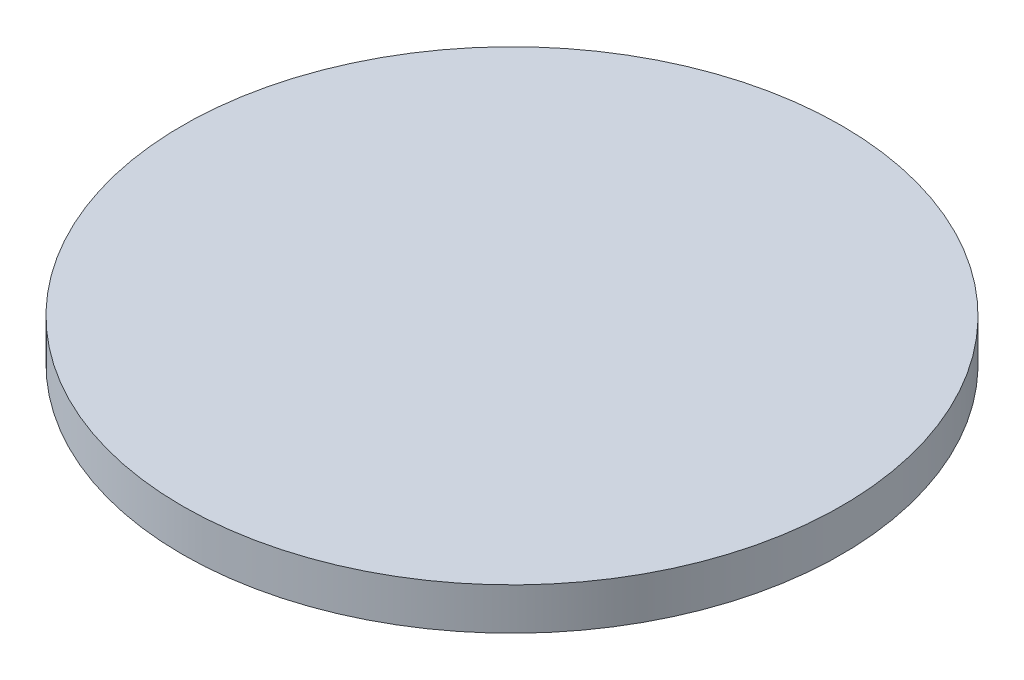
SolidWorks part; units mm, degrees
material "1023 碳钢板 (SS)"
ref_plane "Front Plane" through (0, 0, 0) normal (0, 0, 1) x (1, 0, 0)
ref_plane "Top Plane" through (0, 0, 0) normal (0, 1, 0) x (1, 0, 0)
ref_plane "Right Plane" through (0, 0, 0) normal (1, 0, 0) x (0, 0, -1)
sketch "Sketch1" plane through (0, 210, 0) normal (0, 1, 0) x (1, 0, 0)
  circle A0 centre (0, 0) radius 11.8 construction
  circle A1 centre (0, 0) radius 11.8
extrude "Boss-Extrude1" add sketch "Sketch1" against normal blind 1.5
